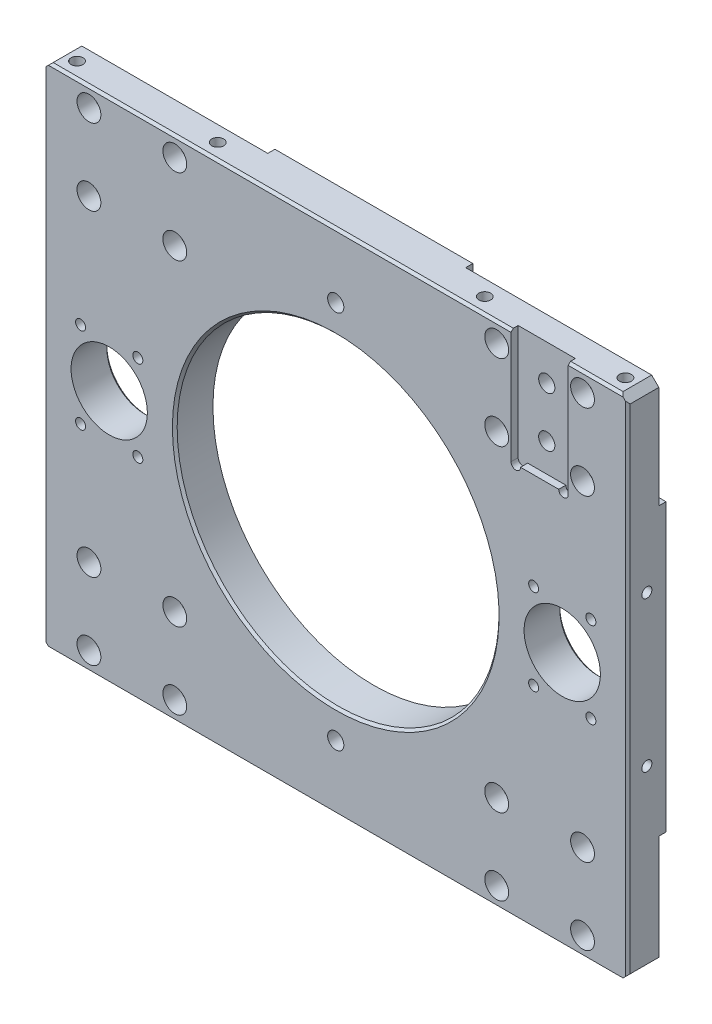
from build123d import *

# Parameters (mm, degrees)
SKETCH1_W                                           = 245
SKETCH1_H                                           = 213
BOSS_EXTRUDE1_DEPTH                                 = 16
CHAMFER1_SIZE                                       = 3
SKETCH3_R                                           = 67.5
CUT_EXTRUDE2_DEPTH                                  = 100
CHAMFER2_SIZE                                       = 1
SKETCH4_R                                           = 16
CUT_EXTRUDE3_DEPTH                                  = 159
CHAMFER3_SIZE                                       = 1
SKETCH5_W                                           = 81
SKETCH5_H                                           = 46
SKETCH5_H_2                                         = 47
CUT_EXTRUDE4_DEPTH                                  = 3
FILLET1_R                                           = 4
HOLE_SIZE_PER_SOCKET_HEAD_CAP_SCREW_TYP_D           = 5.5
HOLE_SIZE_PER_SOCKET_HEAD_CAP_SCREW_TYP_CBORE_D     = 10
HOLE_SIZE_PER_SOCKET_HEAD_CAP_SCREW_TYP_CBORE_DEPTH = 7
M8_TAPPED_HOLE1_D                                   = 6.8
M8_TAPPED_HOLE1_DEPTH                               = 22.25
M8_TAPPED_HOLE1_TIP                                 = 2.042926105
SKETCH10_W                                          = 24
SKETCH10_H                                          = 69.564356815
CUT_EXTRUDE5_DEPTH                                  = 3
SKETCH11_R                                          = 2
CUT_EXTRUDE6_DEPTH                                  = 38
M8_TAPPED_HOLE2_D                                   = 6.8
M6_TAPPED_HOLE1_D                                   = 5
M6_TAPPED_HOLE1_DEPTH                               = 17
M6_TAPPED_HOLE1_TIP                                 = 1.502151548
M5_TAPPED_HOLE1_D                                   = 4.2
M5_TAPPED_HOLE1_DEPTH                               = 14
M5_TAPPED_HOLE1_TIP                                 = 1.2618073
M5_TAPPED_HOLE2_D                                   = 4.2
M5_TAPPED_HOLE2_DEPTH                               = 14
M5_TAPPED_HOLE2_TIP                                 = 1.2618073
M5_TAPPED_HOLE3_D                                   = 4.2
CHAMFER4_SIZE                                       = 1


with BuildPart() as part:
    # Sketch1 → Boss-Extrude1 (new body)
    with BuildSketch(Plane.XY):
        Rectangle(SKETCH1_W, SKETCH1_H)
    extrude(amount=BOSS_EXTRUDE1_DEPTH)

    # Chamfer1
    chamfer1_edges = [part.edges().sort_by_distance(p)[0] for p in [
        (122.5, -106.5, 8),
        (-122.5, -106.5, 8),
        (-122.5, 106.5, 8),
        (122.5, 106.5, 8),
    ]]
    chamfer(chamfer1_edges, length=CHAMFER1_SIZE)

    # Sketch3 → Cut-Extrude2 (cut)
    with BuildSketch(Plane.XY.offset(16)):
        Circle(SKETCH3_R)
    extrude(amount=-CUT_EXTRUDE2_DEPTH, mode=Mode.SUBTRACT)

    # Chamfer2
    chamfer2_edges = [part.edges().sort_by_distance(p)[0] for p in [
        (-67.5, 0, 16),
    ]]
    chamfer(chamfer2_edges, length=CHAMFER2_SIZE)

    # Sketch4 → Cut-Extrude3 (cut)
    with BuildSketch(Plane.XY.offset(16)):
        with Locations((-95, 0)):
            Circle(SKETCH4_R)
        with Locations((95, 0)):
            Circle(SKETCH4_R)
    extrude(amount=-CUT_EXTRUDE3_DEPTH, mode=Mode.SUBTRACT)

    # Chamfer3
    chamfer3_edges = [part.edges().sort_by_distance(p)[0] for p in [
        (0, 106.5, 16),
        (122.5, 0, 16),
        (-122.5, 0, 16),
        (0, -106.5, 16),
    ]]
    chamfer(chamfer3_edges, length=CHAMFER3_SIZE)

    # Sketch5 → Cut-Extrude4 (cut)
    with BuildSketch(Plane(origin=(0, 0, 0), x_dir=(-1, 0, 0), z_dir=(0, 0, -1))):
        with Locations((-82, 83.5)):
            Rectangle(SKETCH5_W, SKETCH5_H)
        with Locations((-82, -83)):
            Rectangle(SKETCH5_W, SKETCH5_H_2)
        with Locations((82, -83)):
            Rectangle(SKETCH5_W, SKETCH5_H_2)
        with Locations((82, 83.5)):
            Rectangle(SKETCH5_W, SKETCH5_H)
    extrude(amount=-CUT_EXTRUDE4_DEPTH, mode=Mode.SUBTRACT)

    # Fillet1
    fillet1_edges = [part.edges().sort_by_distance(p)[0] for p in [
        (-41.5, 60.5, 1.5),
        (-41.5, -59.5, 1.5),
        (41.5, -59.5, 1.5),
        (41.5, 60.5, 1.5),
    ]]
    fillet(fillet1_edges, radius=FILLET1_R)

    # Hole size (per socket head cap screw type)0 (through all)
    with Locations(Plane.XY.offset(16)):
        with Locations((-103.5, -98.5), (-67.5, -98.5), (-67.5, -66.5), (-103.5, -66.5), (67.5, -66.5), (67.5, -98.5), (103.5, -98.5), (103.5, -66.5), (67.5, 98.5), (67.5, 66.5), (103.5, 66.5), (103.5, 98.5), (-103.5, 98.5), (-103.5, 66.5), (-67.5, 66.5), (-67.5, 98.5)):
            CounterBoreHole(HOLE_SIZE_PER_SOCKET_HEAD_CAP_SCREW_TYP_D / 2, HOLE_SIZE_PER_SOCKET_HEAD_CAP_SCREW_TYP_CBORE_D / 2, HOLE_SIZE_PER_SOCKET_HEAD_CAP_SCREW_TYP_CBORE_DEPTH)

    # M8 Tapped Hole1
    with Locations(Plane.XY.offset(16)):
        with Locations((0, 79.5), (0, -79.5)):
            Hole(M8_TAPPED_HOLE1_D / 2, depth=M8_TAPPED_HOLE1_DEPTH)
            with Locations((0, 0, -(M8_TAPPED_HOLE1_DEPTH + M8_TAPPED_HOLE1_TIP / 2))):  # 118° drill point
                Cone(0, M8_TAPPED_HOLE1_D / 2, M8_TAPPED_HOLE1_TIP, mode=Mode.SUBTRACT)

    # Sketch10 → Cut-Extrude5 (cut)
    with BuildSketch(Plane.XY.offset(16)):
        with Locations((85.5, 93.282178407)):
            Rectangle(SKETCH10_W, SKETCH10_H)
    extrude(amount=-CUT_EXTRUDE5_DEPTH, mode=Mode.SUBTRACT)

    # Sketch11 → Cut-Extrude6 (cut)
    with BuildSketch(Plane.XY.offset(13)):
        with Locations((75.5, 58.5)):
            Circle(SKETCH11_R)
        with Locations((95.5, 58.5)):
            Circle(SKETCH11_R)
    extrude(amount=CUT_EXTRUDE6_DEPTH, mode=Mode.SUBTRACT)

    # M8 Tapped Hole2 (through all)
    with Locations(Plane.XY.offset(13)):
        with Locations((85.5, 70.5), (85.5, 91.5)):
            Hole(M8_TAPPED_HOLE2_D / 2)

    # M6 Tapped Hole1
    with Locations(Plane(origin=(0, 106.5, 0), x_dir=(1, 0, 0), z_dir=(0, 1, 0))):
        with Locations((56, -9.5), (115, -9.5), (-56, -9.5), (-115, -9.5)):
            Hole(M6_TAPPED_HOLE1_D / 2, depth=M6_TAPPED_HOLE1_DEPTH)
            with Locations((0, 0, -(M6_TAPPED_HOLE1_DEPTH + M6_TAPPED_HOLE1_TIP / 2))):  # 118° drill point
                Cone(0, M6_TAPPED_HOLE1_D / 2, M6_TAPPED_HOLE1_TIP, mode=Mode.SUBTRACT)

    # M5 Tapped Hole1
    with Locations(Plane(origin=(122.5, 0, 0), x_dir=(0, 0, -1), z_dir=(1, 0, 0))):
        with Locations((-8, -31.5), (-8, 31.5)):
            Hole(M5_TAPPED_HOLE1_D / 2, depth=M5_TAPPED_HOLE1_DEPTH)
            with Locations((0, 0, -(M5_TAPPED_HOLE1_DEPTH + M5_TAPPED_HOLE1_TIP / 2))):  # 118° drill point
                Cone(0, M5_TAPPED_HOLE1_D / 2, M5_TAPPED_HOLE1_TIP, mode=Mode.SUBTRACT)

    # M5 Tapped Hole2
    with Locations(Plane.ZY.offset(122.5)):
        with Locations((8, 31.5), (8, -31.5)):
            Hole(M5_TAPPED_HOLE2_D / 2, depth=M5_TAPPED_HOLE2_DEPTH)
            with Locations((0, 0, -(M5_TAPPED_HOLE2_DEPTH + M5_TAPPED_HOLE2_TIP / 2))):  # 118° drill point
                Cone(0, M5_TAPPED_HOLE2_D / 2, M5_TAPPED_HOLE2_TIP, mode=Mode.SUBTRACT)

    # M5 Tapped Hole3 (through all)
    with Locations(Plane(origin=(0, 0, 0), x_dir=(-1, 0, 0), z_dir=(0, 0, -1))):
        with Locations((-107, 18), (-83, 18), (-83, -18), (-107, -18), (83, 18), (107, 18), (83, -18), (107, -18)):
            Hole(M5_TAPPED_HOLE3_D / 2)

    # Chamfer4
    chamfer4_edges = [part.edges().sort_by_distance(p)[0] for p in [
        (-111, 0, 0),
        (79, 0, 0),
    ]]
    chamfer(chamfer4_edges, length=CHAMFER4_SIZE)


solid = part.part
